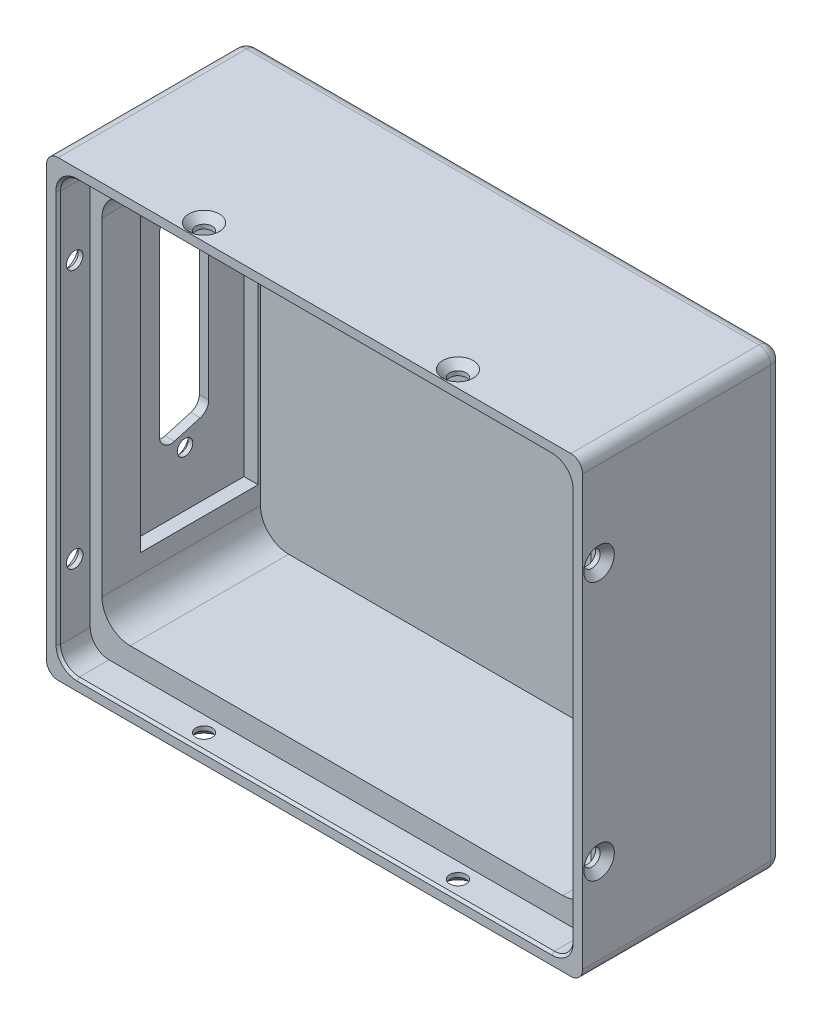
SolidWorks part; units mm, degrees
material "6061 合金"
ref_plane "前视基准面" through (0, 0, 0) normal (0, 0, 1) x (1, 0, 0)
ref_plane "上视基准面" through (0, 0, 0) normal (0, 1, 0) x (1, 0, 0)
ref_plane "右视基准面" through (0, 0, 0) normal (1, 0, 0) x (0, 0, -1)
sketch "草图1" plane through (0, 0, 0) normal (0, 0, 1) x (1, 0, 0)
  line L1 (-57, 48.15) -> (57, 48.15)
  line L2 (-57, 48.15) -> (-57, -48.15)
  line L3 (-57, -48.15) -> (57, -48.15)
  line L4 (57, 48.15) -> (57, -48.15)
  dimension "D1" = 96.3
  dimension "D2" = 114
  dimension "D3" = 57
  dimension "D4" = 48.15
extrude "拉伸1" add sketch "草图1" along normal blind 42.5
sketch "草图2" plane through (0, 0, 42.5) normal (0, 0, 1) x (1, 0, 0)
  line L1 (-52, 40.9) -> (52, 40.9)
  line L2 (-52, 40.9) -> (-52, -40.9)
  line L3 (-52, -40.9) -> (52, -40.9)
  line L4 (52, 40.9) -> (52, -40.9)
  dimension "D1" = 81.8
  dimension "D2" = 40.9
  dimension "D3" = 104
  dimension "D4" = 52
extrude "切除-拉伸1" cut sketch "草图2" against normal blind 40.5
sketch "草图3" plane through (0, 0, 42.5) normal (0, 0, 1) x (1, 0, 0)
  line L1 (-54.5, 45.75) -> (54.5, 45.75)
  line L2 (-54.5, 45.75) -> (-54.5, -45.75)
  line L3 (-54.5, -45.75) -> (54.5, -45.75)
  line L4 (54.5, 45.75) -> (54.5, -45.75)
  dimension "D1" = 91.5
  dimension "D2" = 109
  dimension "D3" = 54.5
  dimension "D4" = 45.75
extrude "切除-拉伸2" cut sketch "草图3" against normal blind 6.8
fillet "圆角1" radius 2.5 8 edges at (0, -48.15, 0) (-57, 0, 0) (57, 0, 0) (0, 48.15, 0) (57, 48.15, 21.25) (57, -48.15, 21.25) (-57, -48.15, 21.25) (-57, 48.15, 21.25)
fillet "圆角2" radius 4 4 edges at (54.5, 45.75, 39.1) (-54.5, 45.75, 39.1) (-54.5, -45.75, 39.1) (54.5, -45.75, 39.1)
fillet "圆角3" radius 6 4 edges at (-52, 40.9, 18.85) (-52, -40.9, 18.85) (52, 40.9, 18.85) (52, -40.9, 18.85)
hole_wizard "孔1" positions "3D草图1" profile "草图5" legacy
sketch3d "3D草图1"
  line L0 (54.5, 48.15, 42.5) -> (-54.5, 48.15, 42.5) construction
  point P0 (27, 48.15, 39)
  point P2 (16.4782, 48.15, 42.5)
  dimension "D1" = 3.5
sketch "草图5" plane through (27, 48.15, 39) normal (1, 0, 0) x (0, 0, 1)
  line L0 (0, 0) -> (0, 10)
  line L1 (0, 10) -> (1.75, 10)
  line L2 (1.75, 10) -> (1.75, 1.5)
  line L3 (1.75, 1.5) -> (3.25, 0)
  line L4 (3.25, 0) -> (0, 0)
  line L5 (0, -6.4453) -> (0, 115.525) construction
  line L6 (-1.75, 1.5) -> (-3.25, 0) construction
  dimension "眻噤" = 3.5
  dimension "旮僅" = 10
  dimension "袪諧褒僅" = 90
  dimension "袪諧眻噤" = 6.5
pattern_linear "阵列(线性)1" count 2 spacing 54 along (-1, 0, 0) of "孔1"
mirror "镜向1" about plane through (0, 0, 0) normal (0, 1, 0) of "孔1", "阵列(线性)1"
hole_wizard "孔2" positions "3D草图2" profile "草图6" legacy
sketch3d "3D草图2"
  line L0 (-57, 45.65, 42.5) -> (-57, -45.65, 42.5) construction
  point P0 (-57, 27.5, 39)
  dimension "D1" = 3.5
sketch "草图6" plane through (-57, 27.5, 39) normal (0, 1, 0) x (0, 0, 1)
  line L0 (0, 0) -> (0, 10)
  line L1 (0, 10) -> (1.75, 10)
  line L2 (1.75, 10) -> (1.75, 1.5)
  line L3 (1.75, 1.5) -> (3.25, 0)
  line L4 (3.25, 0) -> (0, 0)
  line L5 (0, -6.4453) -> (0, 115.525) construction
  line L6 (-1.75, 1.5) -> (-3.25, 0) construction
  dimension "眻噤" = 3.5
  dimension "旮僅" = 10
  dimension "袪諧褒僅" = 90
  dimension "袪諧眻噤" = 6.5
pattern_linear "阵列(线性)2" count 2 spacing 55 along (0, -1, 0) of "孔2"
mirror "镜向2" about plane through (0, 0, 0) normal (1, 0, 0) of "孔2", "阵列(线性)2"
sketch "草图7" plane through (-57, 0, 0) normal (-1, 0, 0) x (0, 0, 1)
  line L0 (10, 23.15) -> (10, -14.85)
  line L1 (10, -14.85) -> (20.5, -17.85)
  line L2 (20.5, -17.85) -> (20.5, 26.15)
  line L3 (20.5, 26.15) -> (10, 23.15)
  line L4 (0, -45.65) -> (0, 45.65) construction
  line L5 (2.5, 48.15) -> (42.5, 48.15) construction
  dimension "D1" = 10
  dimension "D2" = 10.5
  dimension "D3" = 44
  dimension "D4" = 38
  dimension "D5" = 22
extrude "切除-拉伸3" cut sketch "草图7" against normal blind 6.8
fillet "圆角4" radius 2.5 4 edges at (-54.5, -17.85, 20.5) (-54.5, -14.85, 10) (-54.5, 26.15, 20.5) (-54.5, 23.15, 10)
sketch "草图8" plane through (-52, 0, 0) normal (1, 0, 0) x (0, 0, -1)
  line L0 (-42.5, 48.15) -> (-2.5, 48.15) construction
  line L1 (-27.5, 39.15) -> (-2.5, 39.15)
  line L2 (-27.5, 39.15) -> (-27.5, -30.85)
  line L3 (-27.5, -30.85) -> (-2.5, -30.85)
  line L4 (-2.5, 39.15) -> (-2.5, -30.85)
  line L5 (0, 45.65) -> (0, -45.65) construction
  dimension "D1" = 70
  dimension "D2" = 25
  dimension "D3" = 9
  dimension "D4" = 2.5
extrude "切除-拉伸4" cut sketch "草图8" against normal mid plane 6
hole_wizard "孔3" positions "3D草图3" profile "草图9" legacy
sketch3d "3D草图3"
  line L0 (-54.5, -45.65, 0) -> (-54.5, 45.65, 0) construction
  line L1 (-54.5, 48.15, 2.5) -> (-54.5, 48.15, 42.5) construction
  point P0 (-57, 27.803, 15.0437)
  dimension "D1" = 15.25
  dimension "D2" = 20.5
sketch "草图9" plane through (-57, 27.803, 15.0437) normal (0, 1, 0) x (0, 0, 1)
  line L0 (0, 0) -> (0, 10)
  line L1 (0, 10) -> (1.65, 10)
  line L2 (1.65, 10) -> (1.65, 1)
  line L3 (1.65, 1) -> (2.75, 1)
  line L4 (2.75, 1) -> (2.75, 0)
  line L5 (2.75, 0) -> (0, 0)
  line L6 (0, 110) -> (0, -10) construction
  dimension "眻噤" = 3.3
  dimension "旮僅" = 10
  dimension "翐諧眻噤" = 5.5
  dimension "翐諧旮僅" = 1
pattern_linear "阵列(线性)3" count 2 spacing 47 along (0, -1, 0) of "孔3"
chamfer "倒角1" distance 0.5 angle 45 8 edges at (-53.3284, 44.5784, 42.5) (-54.5, 0, 42.5) (-53.3284, -44.5784, 42.5) (0, -45.75, 42.5) (53.3284, -44.5784, 42.5) (54.5, 0, 42.5) (53.3284, 44.5784, 42.5) (0, 45.75, 42.5)
